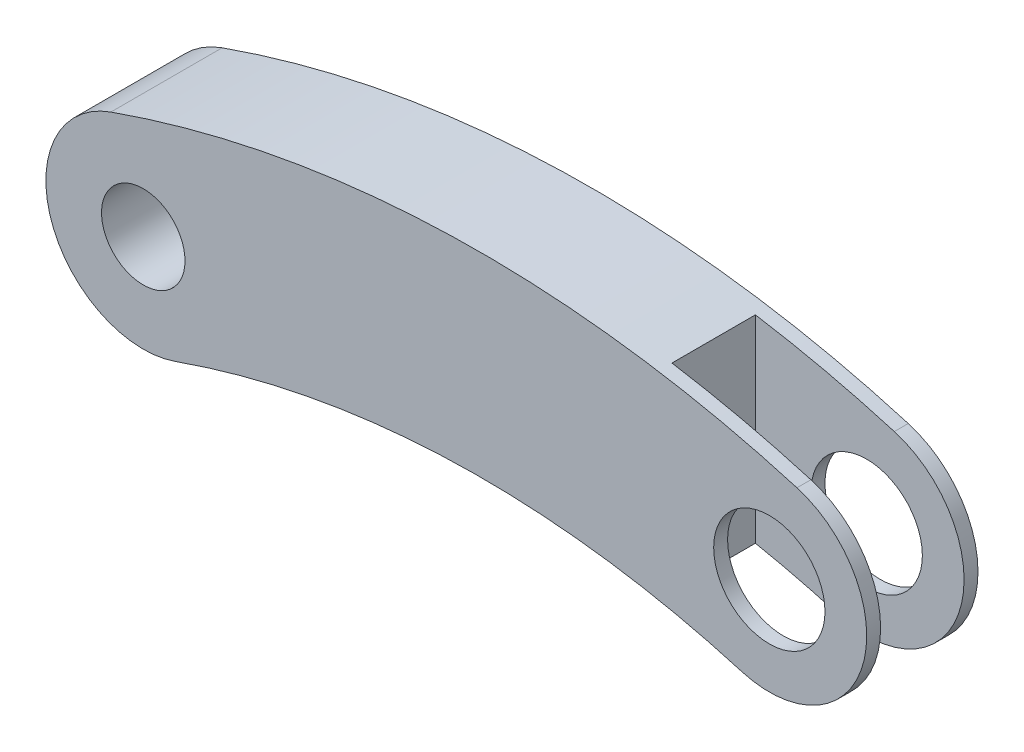
from build123d import *

# Parameters (mm, degrees)
SKETCH1_R               = 3
SKETCH1_R_2             = 4
BOSS_EXTRUDE1_DEPTH     = 8
CUT_EXTRUDE1_DEPTH      = 8
CUT_EXTRUDE1_DEPTH_BACK = 16
SKETCH2_W               = 30
SKETCH2_H               = 6
SCALE1_SCALE            = 0.5


with BuildPart() as part:
    # Sketch1 → Boss-Extrude1 (new body)
    with BuildSketch(Plane.XY):
        with BuildLine():
            ThreePointArc((-50.757929877, -0.048790598), (-26.200561377, 4.481254982), (-1.442861384, 1.219054549))
            ThreePointArc((-1.442861384, 1.219054549), (3.282989256, -7.479585329), (-5.415650622, -12.205435969))
            ThreePointArc((-5.415650622, -12.205435969), (-25.840753116, -9.514120612), (-46.100582129, -13.251408215))
            ThreePointArc((-46.100582129, -13.251408215), (-55.030564812, -8.978773281), (-50.757929877, -0.048790598))
        make_face()
        with Locations((-48.429256003, -6.650099407)):
            Circle(SKETCH1_R, mode=Mode.SUBTRACT)
        with Locations((-3.429256003, -5.49319071)):
            Circle(SKETCH1_R_2, mode=Mode.SUBTRACT)
    extrude(amount=BOSS_EXTRUDE1_DEPTH)

    # Sketch2 → Cut-Extrude1 (cut, two sides: drawn at the far end of the back side and taken through both)
    with BuildSketch(Plane(origin=(0, 0, 0), x_dir=(1, 0, 0), z_dir=(0, 1, 0)).offset(-CUT_EXTRUDE1_DEPTH_BACK)):
        with Locations((3.570743997, -4)):
            Rectangle(SKETCH2_W, SKETCH2_H)
    extrude(amount=CUT_EXTRUDE1_DEPTH + CUT_EXTRUDE1_DEPTH_BACK, mode=Mode.SUBTRACT)


with BuildPart() as part_1:
    # Scale1: scaled about (0, 0, 0)
    add(part.part.scale(SCALE1_SCALE))


solid = part_1.part
